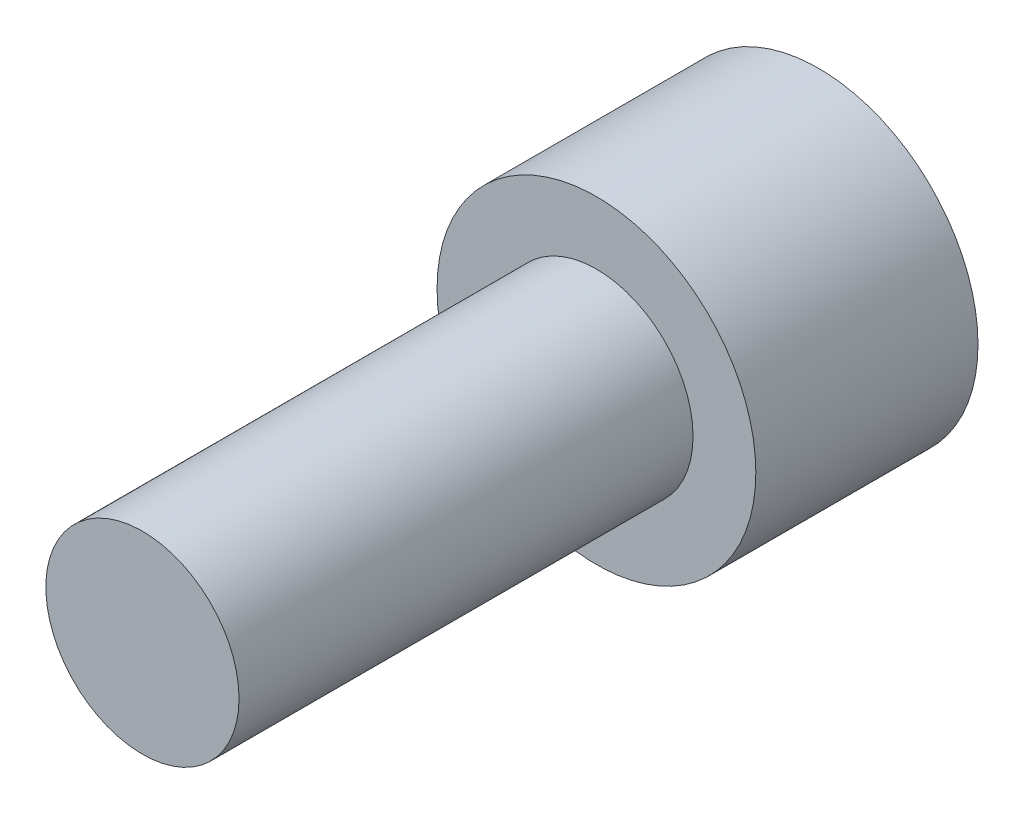
SolidWorks part; units mm, degrees
material "AISI 1045 钢，冷拔"
ref_plane "前视基准面" through (0, 0, 0) normal (0, 0, 1) x (1, 0, 0)
ref_plane "上视基准面" through (0, 0, 0) normal (0, 1, 0) x (1, 0, 0)
ref_plane "右视基准面" through (0, 0, 0) normal (1, 0, 0) x (0, 0, -1)
other "Configuration Table"
sketch "草图1" plane through (0, 0, 0) normal (0, 0, 1) x (1, 0, 0)
  circle A0 centre (0, 0) radius 1.65
  dimension "D1" = 3.3
extrude "凸台-拉伸1" add sketch "草图1" along normal blind 2.3
sketch "草图2" plane through (0, 0, 2.3) normal (0, 0, 1) x (1, 0, 0)
  circle A0 centre (0, 0) radius 1
  dimension "D1" = 2
extrude "凸台-拉伸2" add sketch "草图2" along normal blind 4.7
